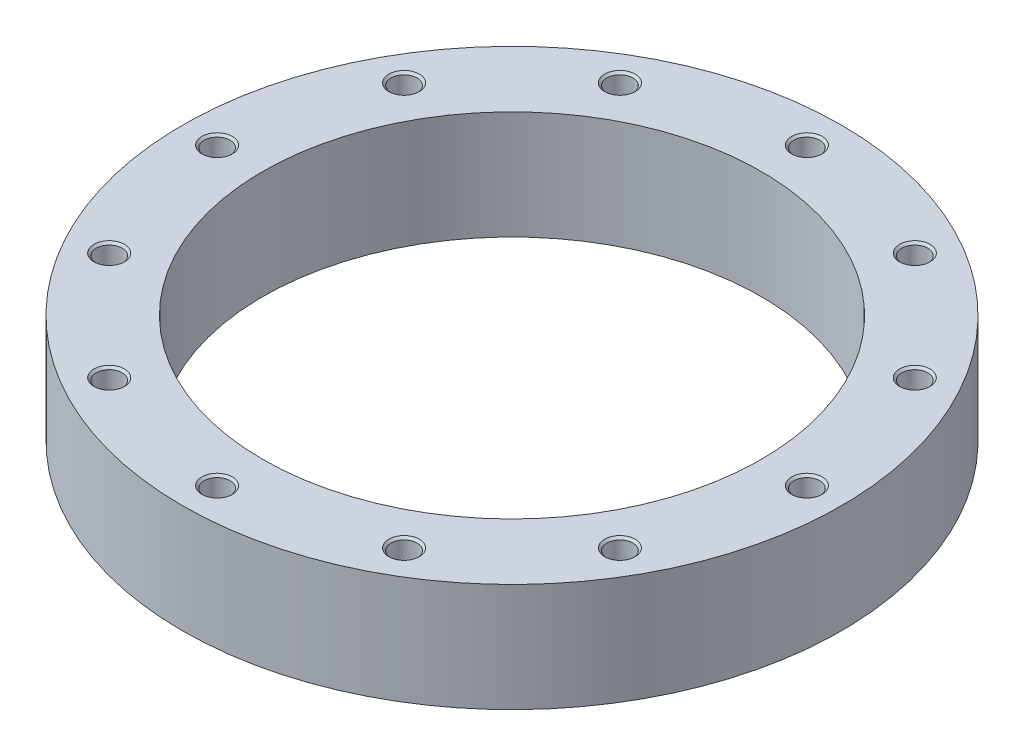
from build123d import *

# Parameters (mm, degrees)
SKETCH1_R                    = 152
BOSS_EXTRUDE1_DEPTH          = 50
M14_TAPPED_HOLE1_D           = 12
M14_TAPPED_HOLE1_CSINK_D     = 14.05
M14_TAPPED_HOLE1_CSINK_ANGLE = 90
SKETCH4_R                    = 115
BOSS_EXTRUDE2_DEPTH          = 5
M14_TAPPED_HOLE2_D           = 12
M14_TAPPED_HOLE2_CSINK_D     = 14.05
M14_TAPPED_HOLE2_CSINK_ANGLE = 90
SKETCH8_R                    = 115
CUT_EXTRUDE1_DEPTH           = 222.885105404


with BuildPart() as part:
    # Sketch1 → Boss-Extrude1 (new body)
    with BuildSketch(Plane(origin=(0, 0, 0), x_dir=(1, 0, 0), z_dir=(0, 1, 0))):
        with Locations(Location((0, 0, 0), (0, 0, 270))):
            Circle(SKETCH1_R)
    extrude(amount=BOSS_EXTRUDE1_DEPTH)

    # M14 Tapped Hole1 (through all)
    with Locations(Plane(origin=(0, 50, 0), x_dir=(1, 0, 0), z_dir=(0, 1, 0))):
        with Locations((-68, 117.779454915), (0, 136), (68, 117.779454915), (117.779454915, 68), (136, 0), (117.779454915, -68), (68, -117.779454915), (0, -136), (-68, -117.779454915), (-117.779454915, -68), (-136, 0), (-117.779454915, 68)):
            CounterSinkHole(M14_TAPPED_HOLE1_D / 2, M14_TAPPED_HOLE1_CSINK_D / 2, counter_sink_angle=M14_TAPPED_HOLE1_CSINK_ANGLE)

    # Sketch4 → Boss-Extrude2 (add)
    with BuildSketch(Plane(origin=(0, 50, 0), x_dir=(1, 0, 0), z_dir=(0, 1, 0))):
        with Locations(Location((0, 0, 0), (0, 0, 270))):
            Circle(SKETCH4_R)
    extrude(amount=BOSS_EXTRUDE2_DEPTH)

    # M14 Tapped Hole2 (through all)
    with Locations(Plane(origin=(0, 55, 0), x_dir=(1, 0, 0), z_dir=(0, 1, 0))):
        with Locations((-44, 76.210235533), (0, 88), (44, 76.210235533), (76.210235533, 44), (88, 0), (76.210235533, -44), (44, -76.210235533), (0, -88), (-44, -76.210235533), (-76.210235533, -44), (-88, 0), (-76.210235533, 44)):
            CounterSinkHole(M14_TAPPED_HOLE2_D / 2, M14_TAPPED_HOLE2_CSINK_D / 2, counter_sink_angle=M14_TAPPED_HOLE2_CSINK_ANGLE)

    # Sketch8 → Cut-Extrude1 (cut, through all)
    with BuildSketch(Plane(origin=(0, 55, 0), x_dir=(1, 0, 0), z_dir=(0, 1, 0))):
        with Locations(Location((0, 0, 0), (0, 0, 270))):
            Circle(SKETCH8_R)
    extrude(amount=-CUT_EXTRUDE1_DEPTH, mode=Mode.SUBTRACT)


solid = part.part
